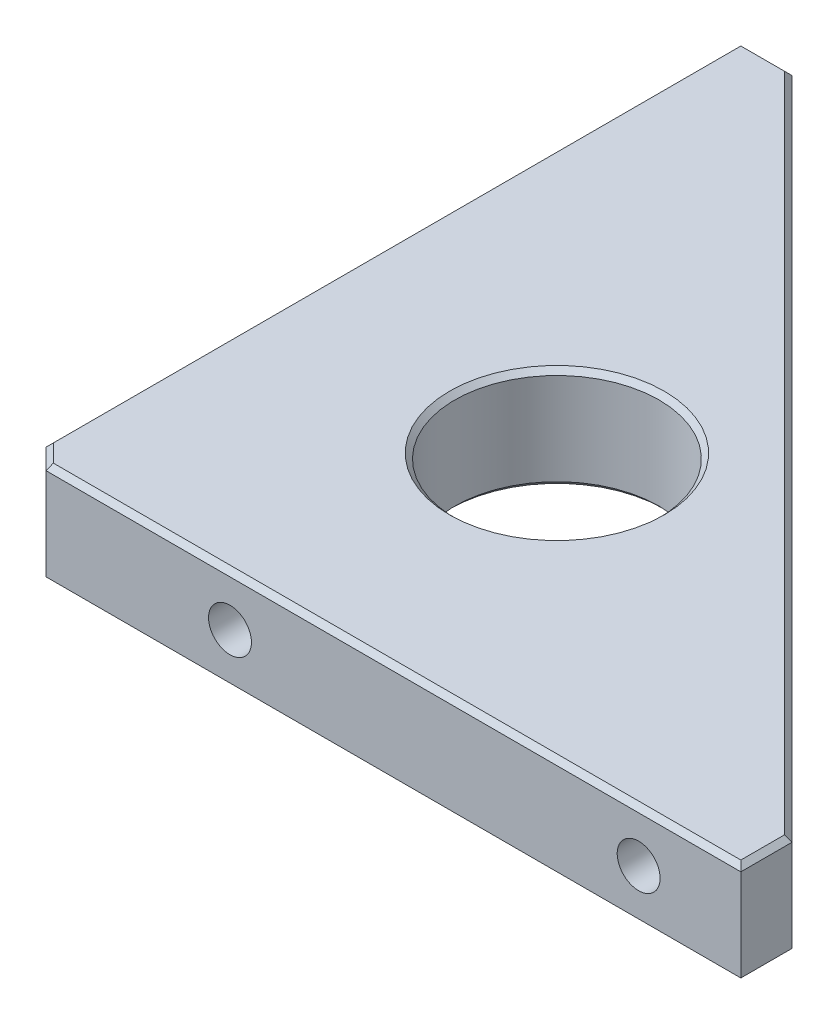
from build123d import *

# Parameters (mm, degrees)
EXTRUDE_1_DEPTH        = 5
CHAMFER_1_SIZE         = 2
HOLE_WIZARD_M5_1_D     = 4.2
HOLE_WIZARD_M5_1_DEPTH = 12.4
HOLE_WIZARD_M5_1_TIP   = 1.2618073
HOLE_WIZARD_M5_2_D     = 4.2
HOLE_WIZARD_M5_2_DEPTH = 12.4
HOLE_WIZARD_M5_2_TIP   = 1.2618073
SKETCH_6_R             = 10
CUT_EXTRUDE_1_DEPTH    = 100.498743711
CHAMFER_2_SIZE         = 0.5


with BuildPart() as part:
    # 草图1 → 凸台-拉伸1 (new, symmetric)
    with BuildSketch(Plane(origin=(0, 0, 0), x_dir=(1, 0, 0), z_dir=(0, 1, 0))):
        Polygon((0, 0), (0, 70), (5, 70), (70, 5), (70, 0), align=None)
    extrude(amount=EXTRUDE_1_DEPTH, both=True)

    # 倒角1
    chamfer_1_edges = [part.edges().sort_by_distance(p)[0] for p in [
        (0, 0, 0),
    ]]
    chamfer(chamfer_1_edges, length=CHAMFER_1_SIZE)

    # M5 螺纹孔1
    with Locations(Plane.XY):
        with Locations((60, 0), (20, 0)):
            Hole(HOLE_WIZARD_M5_1_D / 2, depth=HOLE_WIZARD_M5_1_DEPTH)
            with Locations((0, 0, -(HOLE_WIZARD_M5_1_DEPTH + HOLE_WIZARD_M5_1_TIP / 2))):  # 118° drill point
                Cone(0, HOLE_WIZARD_M5_1_D / 2, HOLE_WIZARD_M5_1_TIP, mode=Mode.SUBTRACT)

    # M5 螺纹孔2
    with Locations(Plane.ZY):
        with Locations((-19.054479799, 0), (-59.054479799, 0)):
            Hole(HOLE_WIZARD_M5_2_D / 2, depth=HOLE_WIZARD_M5_2_DEPTH)
            with Locations((0, 0, -(HOLE_WIZARD_M5_2_DEPTH + HOLE_WIZARD_M5_2_TIP / 2))):  # 118° drill point
                Cone(0, HOLE_WIZARD_M5_2_D / 2, HOLE_WIZARD_M5_2_TIP, mode=Mode.SUBTRACT)

    # 草图6 → 切除-拉伸1 (cut, through all)
    with BuildSketch(Plane.XZ.offset(5)):
        with Locations(Location((26, -26, 0), (0, 0, 270))):
            Circle(SKETCH_6_R)
    extrude(amount=-CUT_EXTRUDE_1_DEPTH, mode=Mode.SUBTRACT)

    # 倒角2
    chamfer_2_edges = [part.edges().sort_by_distance(p)[0] for p in [
        (37.5, 5, -37.5),
        (2.5, 5, -70),
        (36, -5, 0),
        (0, 5, -36),
        (36, 5, 0),
        (1, -5, -1),
        (1, 5, -1),
        (26, 5, -16),
        (26, -5, -16),
        (0, -5, -36),
        (2.5, -5, -70),
        (37.5, -5, -37.5),
        (70, -5, -2.5),
        (70, 5, -2.5),
    ]]
    chamfer(chamfer_2_edges, length=CHAMFER_2_SIZE)


solid = part.part
